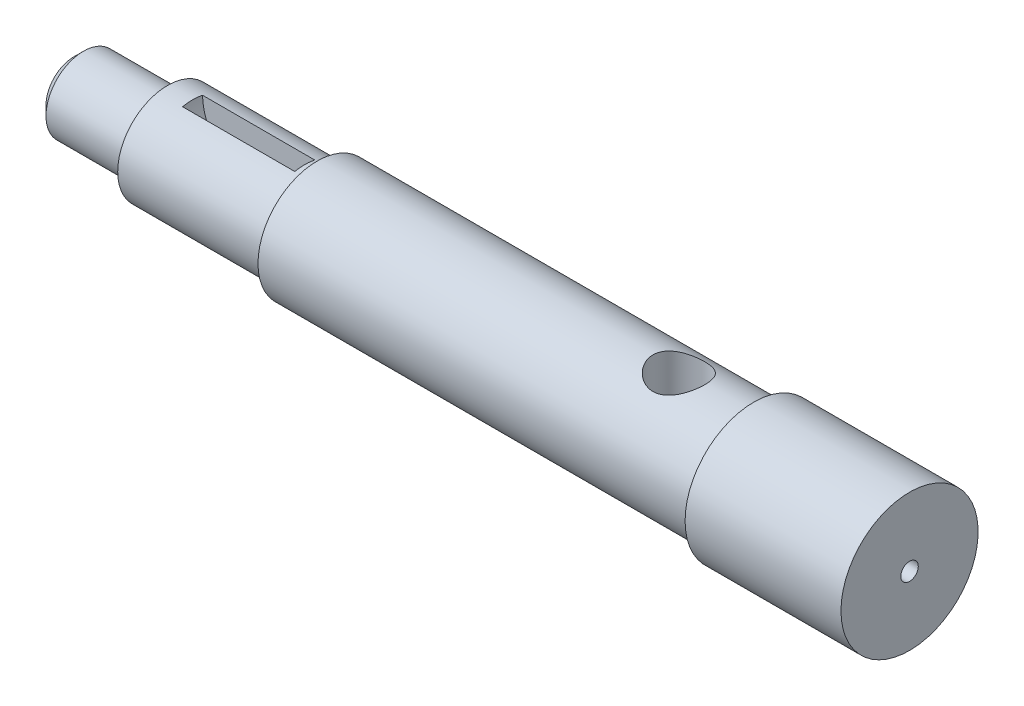
from build123d import *

# Parameters (mm, degrees)
SKETCH2_R               = 1.4
CUT_EXTRUDE1_DEPTH      = 44
CUT_EXTRUDE2_DEPTH      = 84.095495831
CUT_EXTRUDE2_DEPTH_BACK = 84.095495831
SKETCH3_R               = 4.15
SKETCH5_W               = 9
SKETCH5_H               = 3.2
CHAMFER1_SIZE           = 1.5


with BuildPart() as part:
    # Sketch1 → Revolve1 (revolve)
    with BuildSketch(Plane(origin=(0, 0, 0), x_dir=(1, 0, 0), z_dir=(0, 1, 0)), mode=Mode.PRIVATE) as revolve1_sk:
        Polygon((-52.373647469, 0), (-52.373647469, 6), (-37.373647469, 6), (-37.373647469, 8), (-13.373647469, 8), (-13.373647469, 9.5), (56.626352531, 9.5), (56.626352531, 11), (81.626352531, 11), (81.626352531, 0), align=None)
    revolve(revolve1_sk.sketch.rotate(Axis((-52.373647469, 0, 0), (1, 0, 0)), 180), axis=Axis((-52.373647469, 0, 0), (1, 0, 0)))

    # Sketch2 → Cut-Extrude1 (cut)
    with BuildSketch(Plane(origin=(81.626352531, 0, 0), x_dir=(0, 0, -1), z_dir=(1, 0, 0))):
        Circle(SKETCH2_R)
    extrude(amount=-CUT_EXTRUDE1_DEPTH, mode=Mode.SUBTRACT)

    # Sketch3 → Cut-Extrude2 (cut, two sides: drawn at the far end of the back side and taken through both)
    with BuildSketch(Plane(origin=(0, 0, 0), x_dir=(1, 0, 0), z_dir=(0, 1, 0)).offset(-CUT_EXTRUDE2_DEPTH_BACK)):
        with Locations(Location((44.626352531, 0, 0), (0, 0, 270))):
            Circle(SKETCH3_R)
    extrude(amount=CUT_EXTRUDE2_DEPTH + CUT_EXTRUDE2_DEPTH_BACK, mode=Mode.SUBTRACT)

    # Sketch5 → Cut-Revolve3 (revolve, cut)
    with BuildSketch(Plane(origin=(0, 8, 0), x_dir=(-1, 0, 0), z_dir=(0, 1, 0))):
        with Locations((19.873647469, 0)):
            Rectangle(SKETCH5_W, SKETCH5_H)
    revolve(axis=Axis((-24.373647469, 8, 1.6), (0, 0, -1)), mode=Mode.SUBTRACT)

    # Chamfer1
    chamfer1_edges = [part.edges().sort_by_distance(p)[0] for p in [
        (-52.373647469, 0, -6),
    ]]
    chamfer(chamfer1_edges, length=CHAMFER1_SIZE)


solid = part.part
